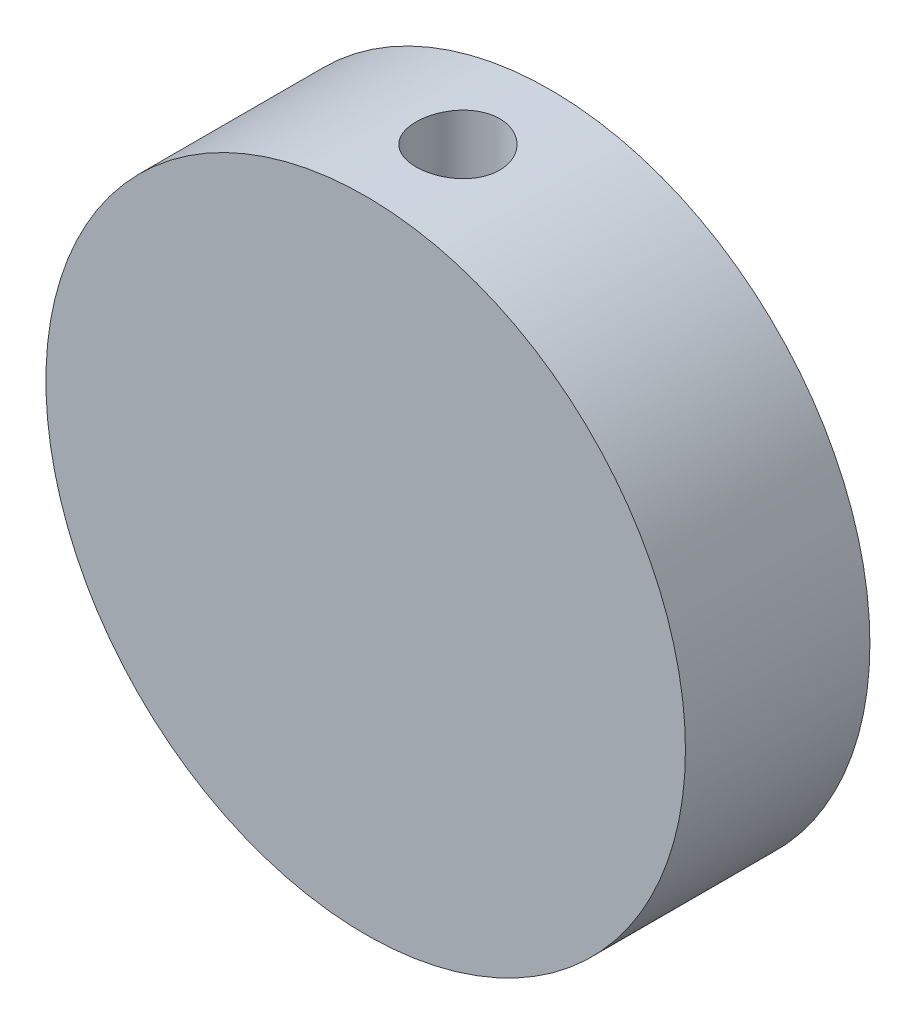
from build123d import *

# Parameters (mm, degrees)
SKETCH1_R           = 26
BOSS_EXTRUDE1_DEPTH = 7.5


with BuildPart() as part:
    # Sketch1 → Boss-Extrude1 (new, symmetric)
    with BuildSketch(Plane.XY):
        with Locations((-106.5, 71.3)):
            Circle(SKETCH1_R)
    extrude(amount=BOSS_EXTRUDE1_DEPTH, both=True)

    # Sketch2 → Cut-Revolve1 (revolve, cut)
    with BuildSketch(Plane.XY):
        Polygon((-106.5, 97.3), (-103.1, 97.3), (-103.1, 87.262990915), (-106.5, 85.3), align=None)
    revolve(axis=Axis((-106.5, 71.3, 0), (0, 1, 0)), mode=Mode.SUBTRACT)


solid = part.part
